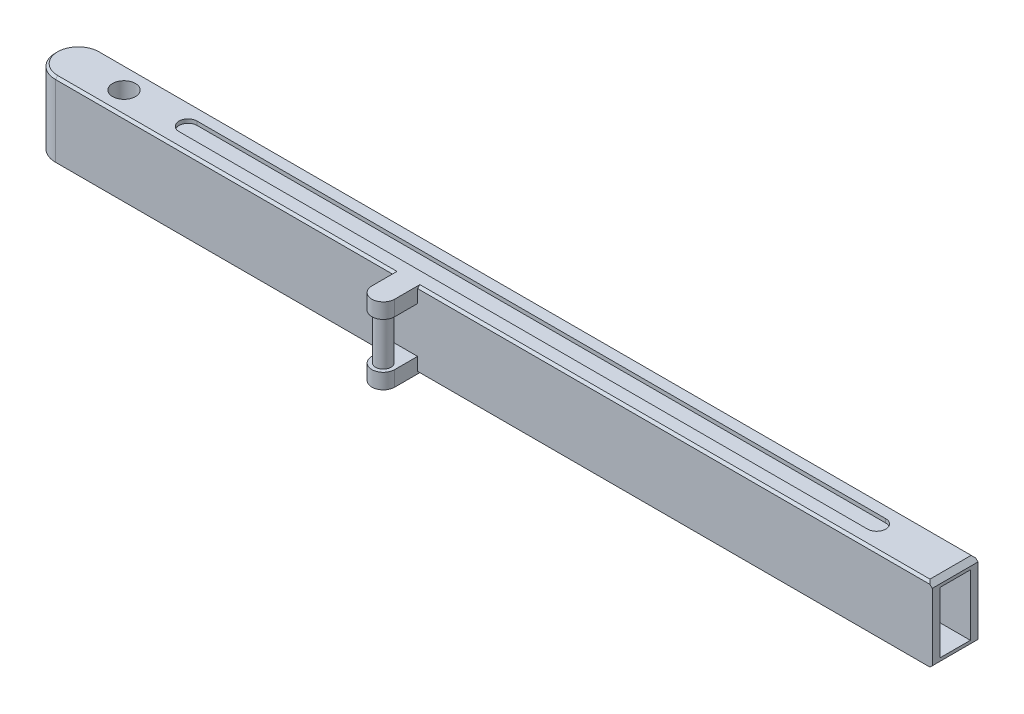
from build123d import *

# Parameters (mm, degrees)
SKETCH1_R           = 150
BOSS_EXTRUDE1_DEPTH = 1000
BOSS_EXTRUDE2_DEPTH = 200
SKETCH4_R           = 100
BOSS_EXTRUDE3_DEPTH = 700
SKETCH5_W           = 400
SKETCH5_H           = 800
CUT_EXTRUDE1_DEPTH  = 10000
CUT_EXTRUDE2_DEPTH  = 50
CHAMFER1_SIZE       = 30
CHAMFER2_SIZE       = 60


with BuildPart() as part:
    # Sketch1 → Boss-Extrude1 (new body)
    with BuildSketch(Plane(origin=(0, 0, 0), x_dir=(1, 0, 0), z_dir=(0, 1, 0))):
        with BuildLine():
            Line((0, 0), (11500, 0))
            Line((11500, 0), (11500, 600))
            Line((11500, 600), (694.445039307, 600))
            Line((694.445039307, 600), (0, 600))
            ThreePointArc((0, 600), (-300, 300), (0, 0))
        make_face()
        with Locations(Location((600, 300, 0), (0, 0, 270))):
            Circle(SKETCH1_R, mode=Mode.SUBTRACT)
    extrude(amount=BOSS_EXTRUDE1_DEPTH)

    # Sketch3 → Boss-Extrude2 (add)
    with BuildSketch(Plane(origin=(0, 1000, 0), x_dir=(1, 0, 0), z_dir=(0, 1, 0))):
        with BuildLine():
            Line((4750, 203.262446468), (4750, -300))
            ThreePointArc((4750, -300), (4600, -450), (4450, -300))
            Line((4450, -300), (4450, 203.262446468))
            ThreePointArc((4450, 203.262446468), (4600, 353.262446468), (4750, 203.262446468))
        make_face()
    boss_extrude2 = extrude(amount=-BOSS_EXTRUDE2_DEPTH)

    # Mirror1: Boss-Extrude2 across plane
    add(boss_extrude2.mirror(Plane.ZX.offset(500)))

    # Sketch4 → Boss-Extrude3 (add)
    with BuildSketch(Plane.XZ.offset(-800)):
        with Locations(Location((4600, 300, 0), (0, 0, 90))):
            Circle(SKETCH4_R)
    extrude(amount=BOSS_EXTRUDE3_DEPTH)

    # Sketch5 → Cut-Extrude1 (cut)
    with BuildSketch(Plane(origin=(11500, 0, 0), x_dir=(0, 0, -1), z_dir=(1, 0, 0))):
        with Locations((300, 500)):
            Rectangle(SKETCH5_W, SKETCH5_H)
    extrude(amount=-CUT_EXTRUDE1_DEPTH, mode=Mode.SUBTRACT)

    # Sketch6 → Cut-Extrude2 (cut)
    with BuildSketch(Plane.XZ):
        with BuildLine():
            Line((1432.066035129, -188.683053799), (10462.796428136, -188.683053799))
            ThreePointArc((10462.796428136, -188.683053799), (10581.914289518, -307.800915181), (10462.796428136, -426.918776563))
            Line((10462.796428136, -426.918776563), (1432.066035129, -426.918776563))
            ThreePointArc((1432.066035129, -426.918776563), (1312.948173747, -307.800915181), (1432.066035129, -188.683053799))
        make_face()
    cut_extrude2 = extrude(amount=-CUT_EXTRUDE2_DEPTH, mode=Mode.SUBTRACT)

    # Mirror2: Cut-Extrude2 across plane
    add(cut_extrude2.mirror(Plane.ZX.offset(500)), mode=Mode.SUBTRACT)

    # Chamfer1
    chamfer1_edges = [part.edges().sort_by_distance(p)[0] for p in [
        (5750, 1000, -600),
        (8125, 1000, 0),
        (8125, 0, 0),
        (-300, 1000, -300),
        (5750, 0, -600),
        (2225, 0, 0),
        (-300, 0, -300),
        (2225, 1000, 0),
    ]]
    chamfer(chamfer1_edges, length=CHAMFER1_SIZE)

    # Chamfer2
    chamfer2_edges = [part.edges().sort_by_distance(p)[0] for p in [
        (11500, 1000, -300),
        (11500, 0, -300),
    ]]
    chamfer(chamfer2_edges, length=CHAMFER2_SIZE)


solid = part.part
